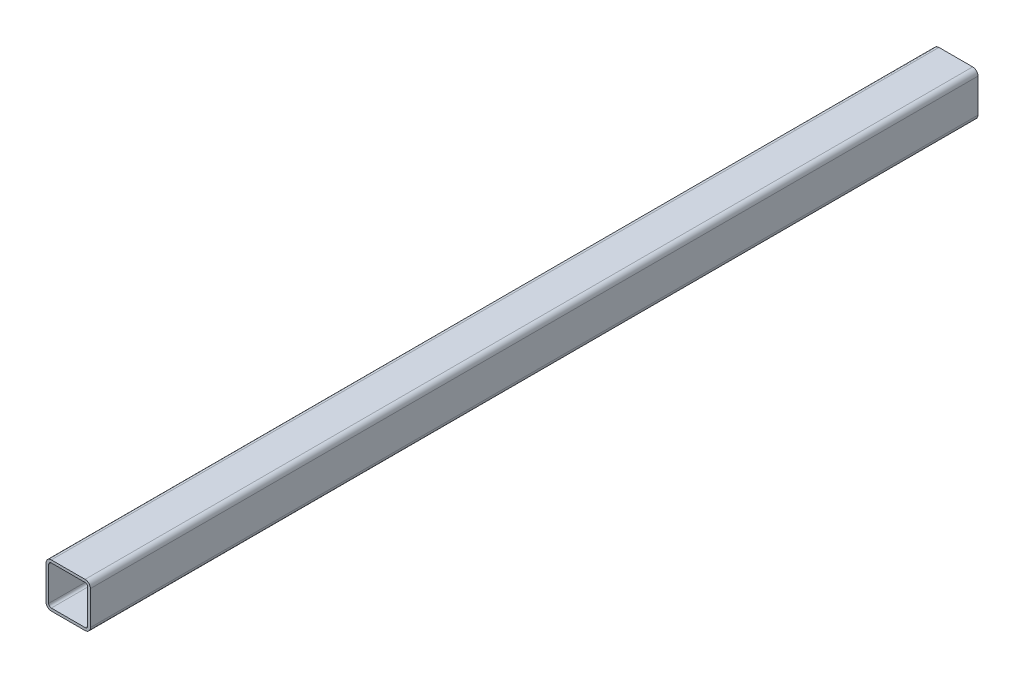
from build123d import *

# Parameters (mm, degrees)
GB_6728_1986_050_X_50_X_3_1_DEPTH = 1000


with BuildPart() as part:
    # Sketch1 → Gb／6728-1986方形空心型钢 050 X 50 X 3(1) (new body)
    with BuildSketch(Plane.YX.offset(-500)):
        with BuildLine():
            Line((-19, -25), (19, -25))
            ThreePointArc((19, -25), (23.242640687, -23.242640687), (25, -19))
            Line((25, -19), (25, 19))
            ThreePointArc((25, 19), (23.242640687, 23.242640687), (19, 25))
            Line((19, 25), (-19, 25))
            ThreePointArc((-19, 25), (-23.242640687, 23.242640687), (-25, 19))
            Line((-25, 19), (-25, -19))
            ThreePointArc((-25, -19), (-23.242640687, -23.242640687), (-19, -25))
        make_face()
        with BuildLine():
            Line((-19, -22), (19, -22))
            ThreePointArc((19, -22), (21.121320344, -21.121320344), (22, -19))
            Line((22, -19), (22, 19))
            ThreePointArc((22, 19), (21.121320344, 21.121320344), (19, 22))
            Line((19, 22), (-19, 22))
            ThreePointArc((-19, 22), (-21.121320344, 21.121320344), (-22, 19))
            Line((-22, 19), (-22, -19))
            ThreePointArc((-22, -19), (-21.121320344, -21.121320344), (-19, -22))
        make_face(mode=Mode.SUBTRACT)
    extrude(amount=GB_6728_1986_050_X_50_X_3_1_DEPTH)


solid = part.part
